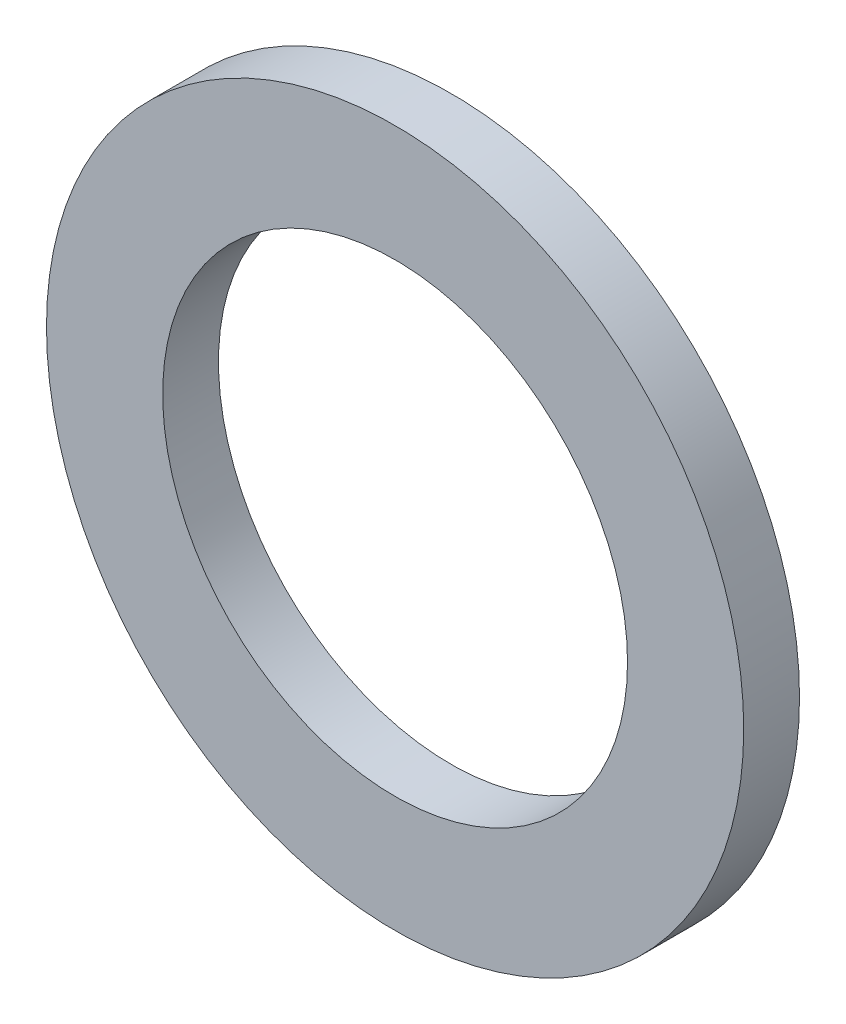
SolidWorks part; units mm, degrees
material "Q235"
ref_plane "Front Plane" through (0, 0, 0) normal (0, 0, 1) x (1, 0, 0)
ref_plane "Top Plane" through (0, 0, 0) normal (0, 1, 0) x (1, 0, 0)
ref_plane "Right Plane" through (0, 0, 0) normal (1, 0, 0) x (0, 0, -1)
sketch "Sketch1" plane through (0, 0, 0) normal (0, 0, 1) x (1, 0, 0)
  circle A0 centre (0, 0) radius 75
  circle A1 centre (0, 0) radius 50
  dimension "D1" = 100
  dimension "D2" = 150
extrude "Boss-Extrude1" add sketch "Sketch1" along normal blind 12
